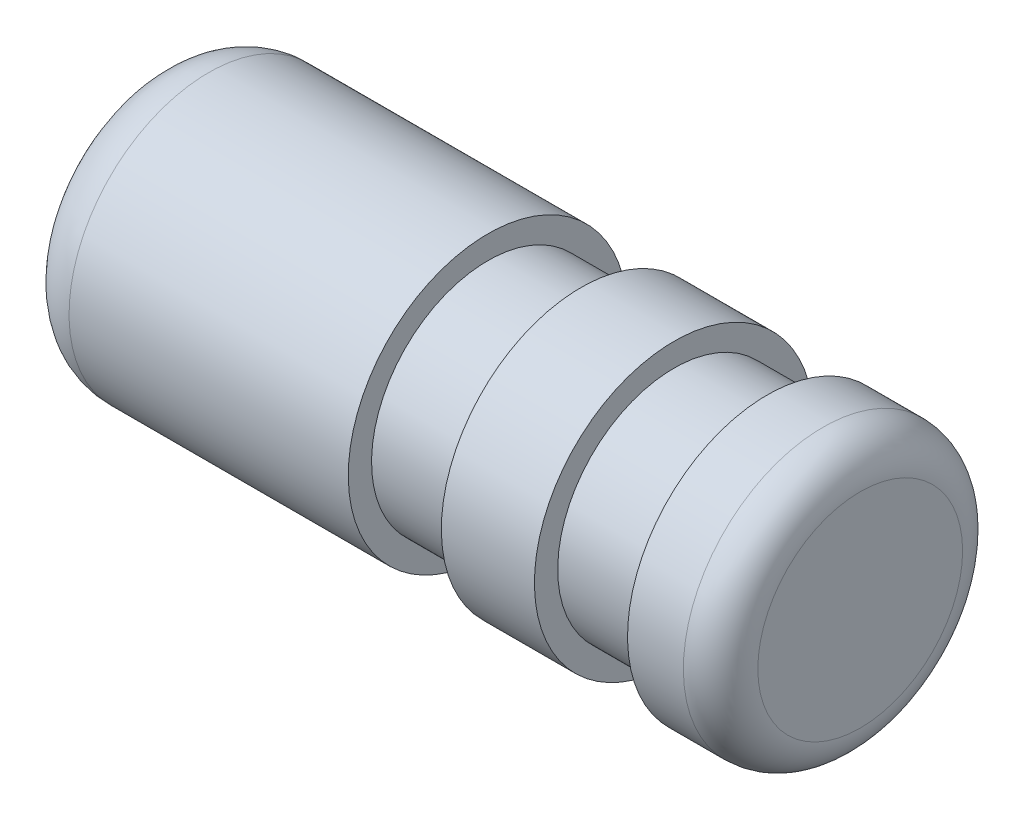
SolidWorks part; units mm, degrees
material "ABS"
ref_plane "前视基准面" through (0, 0, 0) normal (0, 0, 1) x (1, 0, 0)
ref_plane "上视基准面" through (0, 0, 0) normal (0, 1, 0) x (1, 0, 0)
ref_plane "右视基准面" through (0, 0, 0) normal (1, 0, 0) x (0, 0, -1)
sketch "草图1" plane through (0, 0, 0) normal (0, 0, 1) x (1, 0, 0)
  line L0 (-2.5288, 0) -> (2.5288, 0) construction
  line L1 (1.35, 0.75) -> (1.35, 0.625)
  line L2 (-1.65, 0.75) -> (-0.15, 0.75)
  line L3 (-1.95, 0.45) -> (-1.95, 0)
  line L4 (0.35, 0.75) -> (0.85, 0.75)
  line L5 (1.85, 0.55) -> (1.85, 0)
  line L6 (1.35, 0.625) -> (0.85, 0.625)
  line L7 (0.85, 0.625) -> (0.85, 0.75)
  line L8 (-0.15, 0.75) -> (-0.15, 0.625)
  line L9 (-0.15, 0.625) -> (0.35, 0.625)
  line L10 (0.35, 0.625) -> (0.35, 0.75)
  line L11 (1.35, 0.75) -> (1.65, 0.75)
  line L12 (-1.95, 0) -> (1.85, 0)
  arc A0 (-1.65, 0.75) -> (-1.95, 0.45) centre (-1.65, 0.45) ccw
  arc A3 (1.85, 0.55) -> (1.65, 0.75) centre (1.65, 0.55) ccw
  point P3 (0, 0)
  point P11 (-1.95, 0.75)
  point P14 (-1.95, -0.75)
  dimension "D3" = 0.3
  dimension "D8" = 1.25
  dimension "D7" = 0.2
  dimension "D1" = 3.8
  dimension "D2" = 1.5
  dimension "D4" = 0.5
  dimension "D5" = 0.5
  dimension "D6" = 0.5
  dimension "D9" = 1.5
revolve "旋转1" add sketch "草图1" angle 360 about L0
